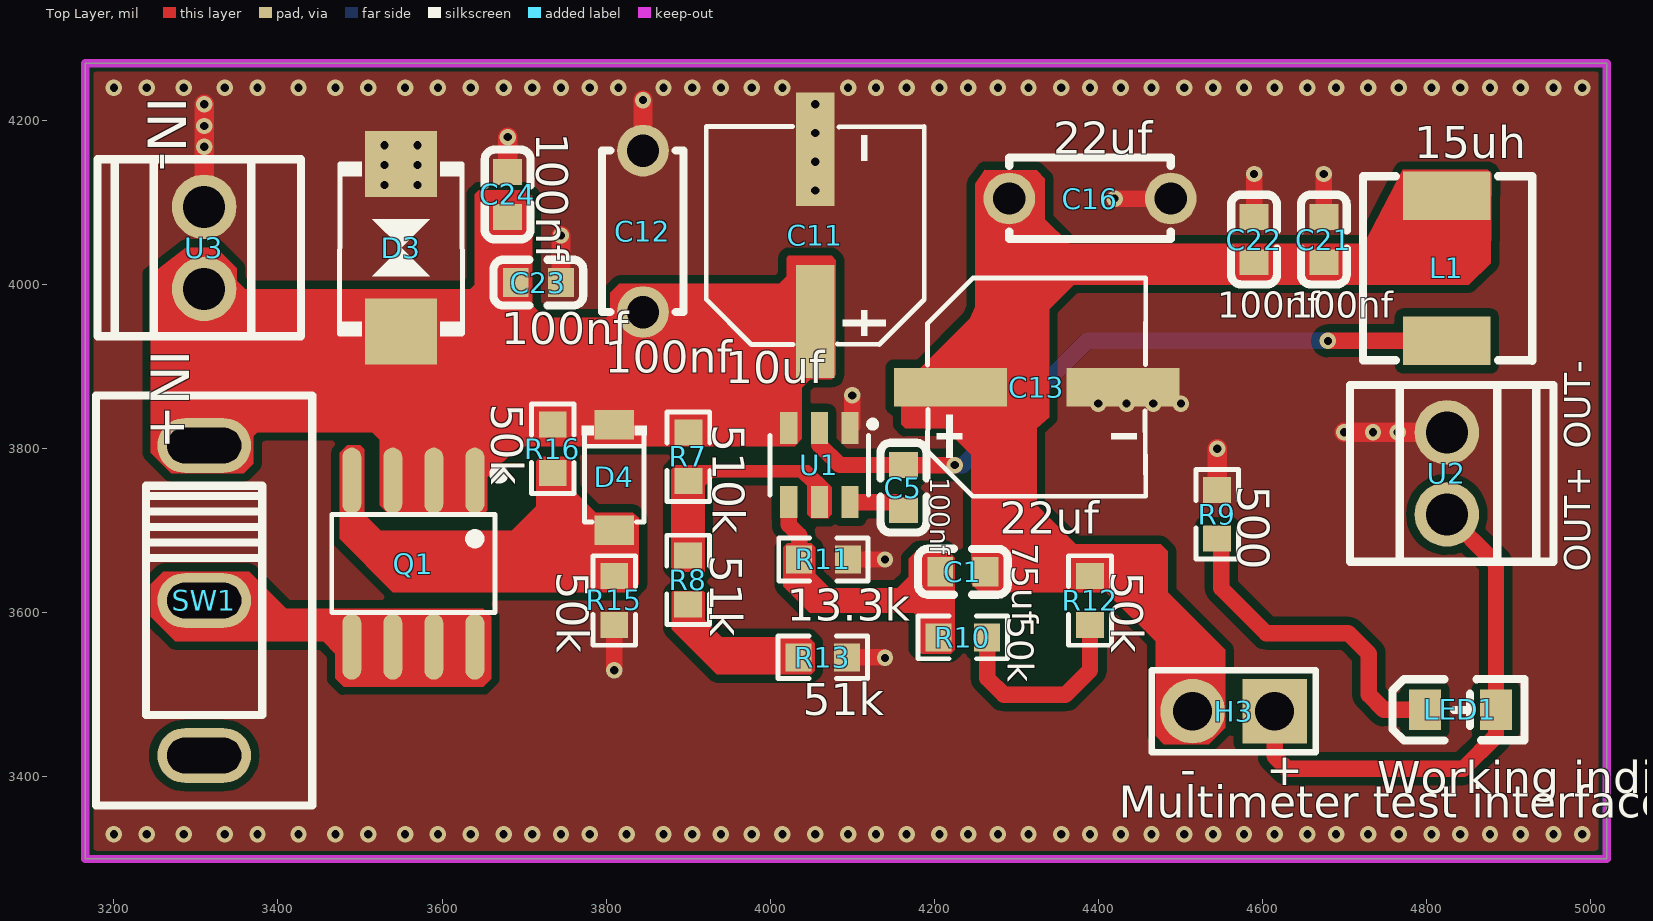
[diagram p0: Top Layer view]
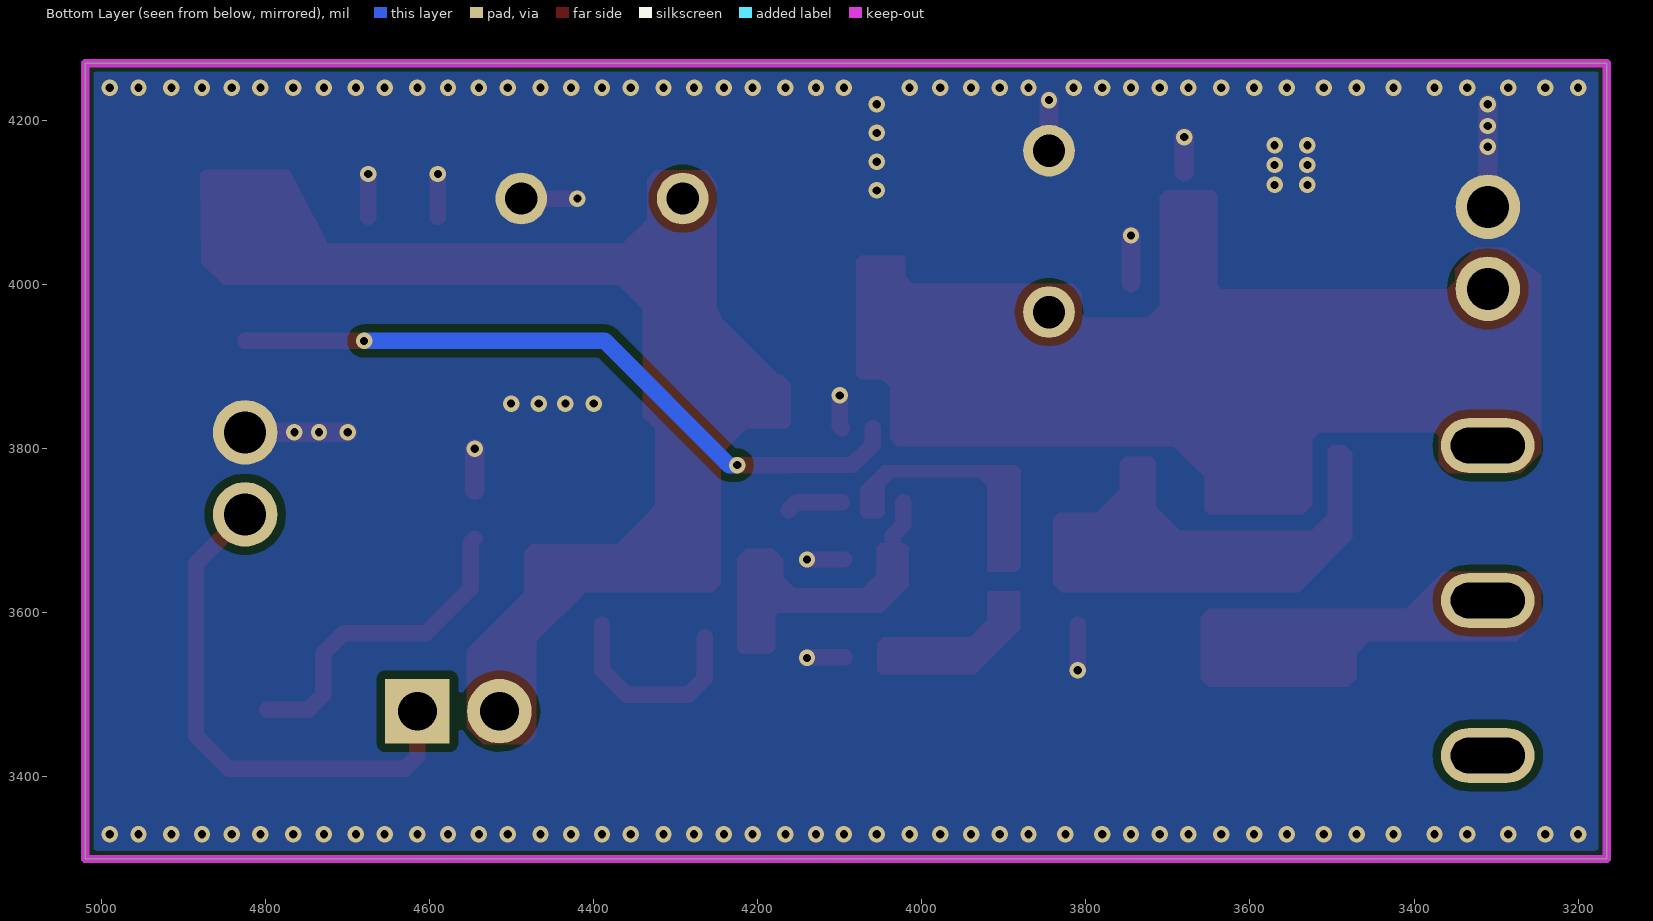
[diagram p1: Bottom Layer view, seen from below]
# Altium PCB MISC52037.pcbdoc
Units mil, origin at the board's own origin, x right, y up, seen from the top; angles counter-clockwise.
Board outline 1855 x 970 mil, 2 copper layers (Top Layer, Bottom Layer), stack 62.206 mil thick; 29 components, 13 nets, 69 pads, 126 vias.

## Layer stack, top to bottom
Top Solder Mask Layer: solder mask 0.394, Dk 3.3
Top Layer: signal copper 1.379
Dielectric1: surface 59.449, FR4, Dk 4.5
Bottom Layer: signal copper 1.378
Bottom Solder Mask Layer: solder mask 0.394, Dk 3.3

## Board outline
3165,4270 3165,3300 5020,3300 5020,4270

## Design rules (kind name [scope] priority, off if disabled: settings)
BoardOutlineClearance copperThickness2oz_1 [All] p2 off: genericclearance=7.99 ignorepadtopadclearanceinfootprint=FALSE except(0: Arc-SplitContinuation Track-SplitContinuation SMDPad-SplitContinuation THPad-SplitContinuation Via-SplitContinuation Fill-SplitContinuation Region-SplitContinuation Poly-SplitContinuation Text-SplitContinuation Hole-SplitContinuation; 5.98: Arc-CutoutEdge SMDPad-CutoutEdge THPad-CutoutEdge Via-CutoutEdge Fill-CutoutEdge Region-CutoutEdge Text-CutoutEdge; 6.93: Hole-OutlineEdge Hole-CutoutEdge; 10: Poly-OutlineEdge Poly-CutoutEdge; 11.81: Arc-OutlineEdge Track-OutlineEdge SMDPad-OutlineEdge THPad-OutlineEdge Via-OutlineEdge Fill-OutlineEdge Region-OutlineEdge Text-OutlineEdge Track-CutoutEdge)
BoardOutlineClearance Plane_innerPlane_1 [All] p4 off: genericclearance=6 ignorepadtopadclearanceinfootprint=FALSE except(0: Arc-SplitContinuation Track-SplitContinuation SMDPad-SplitContinuation THPad-SplitContinuation Via-SplitContinuation Fill-SplitContinuation Region-SplitContinuation Poly-SplitContinuation Text-SplitContinuation Hole-SplitContinuation; 6: SMDPad-CutoutEdge THPad-CutoutEdge Via-CutoutEdge Fill-CutoutEdge Region-CutoutEdge Text-CutoutEdge; 6.93: Hole-OutlineEdge Hole-CutoutEdge; 10: Poly-OutlineEdge Poly-CutoutEdge; 11.8: Arc-OutlineEdge Track-OutlineEdge SMDPad-OutlineEdge THPad-OutlineEdge Via-OutlineEdge Fill-OutlineEdge Region-OutlineEdge Text-OutlineEdge; 11.81: Arc-CutoutEdge Track-CutoutEdge)
BoardOutlineClearance Copper_copperRegion_1 [All] p6 off: genericclearance=6 ignorepadtopadclearanceinfootprint=FALSE except(0: Arc-SplitContinuation Track-SplitContinuation SMDPad-SplitContinuation THPad-SplitContinuation Via-SplitContinuation Fill-SplitContinuation Region-SplitContinuation Poly-SplitContinuation Text-SplitContinuation Hole-SplitContinuation; 6: SMDPad-CutoutEdge THPad-CutoutEdge Via-CutoutEdge Fill-CutoutEdge Region-CutoutEdge Text-CutoutEdge; 6.93: Hole-OutlineEdge Hole-CutoutEdge; 10: Poly-OutlineEdge Poly-CutoutEdge; 11.8: Arc-OutlineEdge Track-OutlineEdge SMDPad-OutlineEdge THPad-OutlineEdge Via-OutlineEdge Fill-OutlineEdge Region-OutlineEdge Text-OutlineEdge; 11.81: Arc-CutoutEdge Track-CutoutEdge)
BoardOutlineClearance copperThickness1oz_1 [All] p8: genericclearance=6 ignorepadtopadclearanceinfootprint=FALSE except(0: Arc-SplitContinuation Track-SplitContinuation SMDPad-SplitContinuation THPad-SplitContinuation Via-SplitContinuation Fill-SplitContinuation Region-SplitContinuation Poly-SplitContinuation Text-SplitContinuation Hole-SplitContinuation; 6: SMDPad-CutoutEdge THPad-CutoutEdge Via-CutoutEdge Fill-CutoutEdge Region-CutoutEdge Text-CutoutEdge; 6.93: Hole-OutlineEdge Hole-CutoutEdge; 10: Poly-OutlineEdge Poly-CutoutEdge; 11.8: Arc-OutlineEdge Track-OutlineEdge SMDPad-OutlineEdge THPad-OutlineEdge Via-OutlineEdge Fill-OutlineEdge Region-OutlineEdge Text-OutlineEdge; 11.81: Arc-CutoutEdge Track-CutoutEdge)
Clearance copperThickness2oz [All] p1 off: gap=7.99 ignorepadtopadclearanceinfootprint=FALSE except(5.98: SMDPad-Track SMDPad-SMDPad THPad-Track SMDPad-THPad THPad-THPad Track-Via SMDPad-Via THPad-Via Via-Via Fill-Track Region-Track Fill-SMDPad Region-SMDPad Fill-THPad Region-THPad Fill-Via Region-Via Fill-Fill Fill-Region Region-Region Arc-Track Arc-SMDPad Arc-THPad Arc-Via Fill-Arc Region-Arc Arc-Arc Text-Track SMDPad-Text Text-THPad Text-Via Fill-Text Region-Text Arc-Text Text-Text; 6.93: Hole-Track Hole-SMDPad Hole-THPad Hole-Via Fill-Hole Region-Hole Hole-Arc Hole-Text; 10: Poly-Track Poly-SMDPad Poly-THPad Poly-Via Poly-Fill Poly-Region Poly-Poly Poly-Arc Poly-Text Poly-Hole)
Clearance Plane_innerPlane [All] p3 off: gap=6 ignorepadtopadclearanceinfootprint=FALSE except(5.98: SMDPad-Track SMDPad-SMDPad THPad-Track SMDPad-THPad THPad-THPad Track-Via SMDPad-Via THPad-Via Via-Via Fill-Track Region-Track Fill-SMDPad Region-SMDPad Fill-THPad Region-THPad Fill-Via Region-Via Fill-Fill Fill-Region Region-Region; 6.93: Hole-Track Hole-SMDPad Hole-THPad Hole-Via Fill-Hole Region-Hole Hole-Arc Hole-Text; 10: Poly-Track Poly-SMDPad Poly-THPad Poly-Via Poly-Fill Poly-Region Poly-Poly Poly-Arc Poly-Text Poly-Hole)
Clearance Copper_copperRegion [All] p5 off: gap=6 ignorepadtopadclearanceinfootprint=FALSE except(5.98: SMDPad-Track SMDPad-SMDPad THPad-Track SMDPad-THPad THPad-THPad Track-Via SMDPad-Via THPad-Via Via-Via Fill-Track Region-Track Fill-SMDPad Region-SMDPad Fill-THPad Region-THPad Fill-Via Region-Via Fill-Fill Fill-Region Region-Region; 6.93: Hole-Track Hole-SMDPad Hole-THPad Hole-Via Fill-Hole Region-Hole Hole-Arc Hole-Text; 10: Poly-Track Poly-SMDPad Poly-THPad Poly-Via Poly-Fill Poly-Region Poly-Poly Poly-Arc Poly-Text Poly-Hole)
Clearance copperThickness1oz [All] p7: gap=6 ignorepadtopadclearanceinfootprint=FALSE except(5.98: SMDPad-Track SMDPad-SMDPad THPad-Track SMDPad-THPad THPad-THPad Track-Via SMDPad-Via THPad-Via Via-Via Fill-Track Region-Track Fill-SMDPad Region-SMDPad Fill-THPad Region-THPad Fill-Via Region-Via Fill-Fill Fill-Region Region-Region; 6.93: Hole-Track Hole-SMDPad Hole-THPad Hole-Via Fill-Hole Region-Hole Hole-Arc Hole-Text; 10: Poly-Track Poly-SMDPad Poly-THPad Poly-Via Poly-Fill Poly-Region Poly-Poly Poly-Arc Poly-Text Poly-Hole)
DiffPairsRouting differentialPair [All] p1: maxlimit=6 minlimit=6 mostfreqgap=6 toplayer_minwidth=5 toplayer_prefwidth=10 toplayer_maxwidth=100 toplayer_mingap=6 toplayer_prefgap=6 toplayer_maxgap=6 bottomlayer_minwidth=5 bottomlayer_prefwidth=10 bottomlayer_maxwidth=100 bottomlayer_mingap=6 bottomlayer_prefgap=6 bottomlayer_maxgap=6 maxuncoupledlength=10
HoleToHoleClearance otherClearance [All] p1: gap=11.81 allowstackedmicrovias=TRUE
Length netLength [All] p1: minlimit=0 maxlimit=0
PasteMaskExpansion pasteMaskExpansion [All] p1: expansion=0
PlaneConnect innerPlane [All] p1: planeconnectstyle=Relief reliefexpansion=20 reliefentries=4 reliefconductorwidth=10 reliefairgap=10
PolygonConnect copperRegion [All] p1: connectstyle=Direct reliefconductorwidth=10 reliefentries=4 polygonreliefangle="90 Angle" airgapwidth=10 via.connectstyle=Relief via.reliefconductorwidth=10 via.reliefentries=4 via.polygonreliefangle="90 Angle" via.airgapwidth=10
RoutingVias viaSize [All] p1: holewidth=10 width=20 viastyle="Through Hole" minholewidth=9 minwidth=19.68 maxholewidth=248.03 maxwidth=393.7
SolderMaskExpansion solderMaskExpansion [IsVia] p1: expansion=-1000 istentingtop=TRUE
SolderMaskExpansion solderMaskExpansion [All] p2: expansion=2 istentingtop=FALSE
Width copperThickness2oz_2 [All] p1 off: maxlimit=100 minlimit=8 preferedwidth=10
Width copperThickness1oz_2 [All] p2: maxlimit=100 minlimit=5 preferedwidth=20

## Components (designator, comment, footprint, x,y, rotation, side; value= is the part's Value field where it differs from the comment)
C1 "75uf" C0603 4235,3650 r0 top
C5 "0.1uf" C0603 4162.56,3752.56 r270 top
C11 "10uf" CAP-SMD_BD6.3-L6.6-W6.6-FD 4055,4060 r90 top
C12 "100nf" CAP-TH_L5.0-W2.5-P5.00-D1.0 3845,4065 r270 top
C13 "22uf" CAP-SMD_BD6.3-L6.6-W6.6-FD 4325,3875 r0 top
C16 "22uf" CAP-TH_L5.0-W2.5-P5.00-D1.0 4390,4105 r180 top
C21 "0.1uf" C0603 4675,4055 r90 top
C22 "0.1uf" C0603 4590,4055 r90 top
C23 "100nf" C0603 3717.44,4002.56 r0 top
C24 "100nf" C0603 3680,4110 r90 top
D3 "SMBJ28CA" SMB_L4.6-W3.6-LS5.4-BI 3550,4045 r270 top
D4 "BZT52C12" SOD-123_L2.7-W1.6-LS3.7-RD 3810,3765 r270 top
H3 "PZ254V-11-02P" HDR-TH_2P-P2.54-V-M 4565,3480 r180 top
L1 "15uH" IND-SMD_L5.7-W5.2_GSM0530 4825,4020 r90 top
LED1 "NCD0805R1" LED0805-RD 4841.62,3481.62 r0 top
Q1 "AO4421" SOIC-8_L4.9-W3.9-P1.27-LS6.0-BL 3565,3660 r180 top
R7 "510kΩ" R0603 3900.34,3790.34 r90 top
R8 "51kΩ" R0603 3900,3640 r90 top
R9 "500Ω" R0603 4545,3720 r270 top
R10 "50kΩ" R0603 4235,3570 r0 top
R11 "13.3kΩ" R0603 4065,3665 r180 top
R12 "50kΩ" R0603 4390,3615 r90 top
R13 "51kΩ" R0603 4064.32,3545.68 r180 top
R15 "50kΩ" R0603 3810,3615 r90 top
R16 "50kΩ" R0603 3735,3800 r90 top
SW1 "SS12D10G4 071" SW-TH_SHOU-HAN_SS12D10G4 3310,3615 r270 top
U1 "GD30DC1354" SOT-23-6_L2.9-W1.7-P0.95-LS2.8-BL 4060,3780 r180 top
U2 "KF128-2.54-2P" CONN-TH_P2.54_KF128-2.54-2P 4825,3770 r90 top
U3 "KF128-2.54-2P" CONN-TH_P2.54_KF128-2.54-2P 3310,4045 r270 top

## Footprints (in the part's own frame and the unit in brackets; to place one, negate y for a bottom-side part, rotate by r counter-clockwise, add the part's x,y. Pads: shape width x height; smd on the part's side, far side on the other; paste and mask are expansions set on the pad)
C0603 [mm]
  rect 0.8x0.9 smd: 1(-0.7,0) 2(0.7,0)
  silkscreen extent -1.39,-0.71 1.39,0.71
CAP-SMD_BD6.3-L6.6-W6.6-FD [mm]
  rect 3.5x1.2 smd: 1(-2.67,0) 2(2.67,0)
  silkscreen extent -3.38,-3.38 3.38,3.38
CAP-TH_L5.0-W2.5-P5.00-D1.0 [mm]
  round 1.6 hole 1: 1(-2.5,0) 2(2.5,0)
  silkscreen extent -2.5,-1.27 2.5,1.25
CONN-TH_P2.54_KF128-2.54-2P [mm]
  round 2 hole 1.3: 1(-1.27,0) 2(1.27,0)
  silkscreen extent -2.74,-3.3 2.74,3
HDR-TH_2P-P2.54-V-M [mm]
  rect 2x2 hole 1.2: 1(-1.27,0)
  round 2 hole 1.2: 2(1.27,0)
  silkscreen extent -2.54,-1.27 2.54,1.27
IND-SMD_L5.7-W5.2_GSM0530 [mm]
  rect 1.5x2.7 smd: 1(-2.25,0) 2(2.25,0)
  silkscreen extent -2.86,-2.64 2.85,2.6
LED0805-RD [mm]
  rect 1x1.25 smd: 1(-1.1,0) 2(1.1,0)
  silkscreen extent -2.1,-0.95 1.98,0.96
R0603 [mil]
  rect 31.75x34.02 smd paste-3937.01 mask+2: 1(-29.66,0) 2(29.66,0)
  silkscreen extent -55,-26 55,26
SMB_L4.6-W3.6-LS5.4-BI [mil]
  rect 80.61x88.23 smd: 1(-102.02,0) 2(102.02,0)
  silkscreen extent -105,-75 108,75
SOD-123_L2.7-W1.6-LS3.7-RD [mm]
  rect 0.91x1.22 smd: 1(-1.635,0) 2(1.635,0)
  silkscreen extent -1.6,-1 1.38,1
SOIC-8_L4.9-W3.9-P1.27-LS6.0-BL [mm]
  oval 0.588x2.045 smd: 1(-1.905,-2.57) 2(-0.635,-2.57) 3(0.635,-2.57) 4(1.905,-2.57) 5(1.905,2.57) 6(0.635,2.57) 7(-0.635,2.57) 8(-1.905,2.57)
  silkscreen extent -2.8,-2.92 2.53,1.52
SOT-23-6_L2.9-W1.7-P0.95-LS2.8-BL [mm]
  rect 0.532x0.99 smd paste+0 mask+0.102: 1(-0.95,-1.145) 2(0,-1.145) 3(0.95,-1.145) 4(0.95,1.145) 5(0,1.145) 6(-0.95,1.145)
  silkscreen extent -1.75,-1.37 1.53,0.93
SW-TH_SHOU-HAN_SS12D10G4 [mm]
  oval 1.7x2.9 hole 1.1 slot 2.3 at 90 deg paste+0 mask+0.05: 1(-4.8,0) 2(0,0) 3(4.8,0)
  silkscreen extent -6.35,-3.35 6.35,3.35

## Via types
v1: diameter 20, hole 10, Top Layer to Bottom Layer, 126 vias

## Nets (pads, with @x,y where several pads share a name; then routed paths per layer and width w, separated by ;. In a path a pad name is that pad's centre, name@x,y a point inside that pad or via, vN(x,y) a via of type N, cw(c..) or ccw(c..) an arc to the next point about the centre after c; other vN are vias at no path point)
24V: C11.1 C12.2 C23.1 C24.1 D3.2 D4.1 Q1.1 Q1.2 Q1.3 R7.2 R16.2 SW1.1 U1.3 U3.2
$1N1: Q1.5 Q1.6 Q1.7 Q1.8 SW1.2
$1N10: LED1.1 R9.2 | length 401.5
  Top Layer w20: R9.2 4550,3685.34 4550,3630 4605,3575 4705,3575 4730,3550 4730,3500 4748.38,3481.62 LED1.1
$1N13: R7.1 R8.2 U1.5
$1N14: C5.2 U1.6 | length 69.3
  Top Layer w20: U1.6 4152.64,3734.92 C5.2
$1N17: C1.2 C13.1 C16.2 C21.1 C22.1 H3.2 L1.2 R12.2
$1N19: R10.2 R12.1 | length 251.2
  Top Layer w20: R10.2 4264.66,3520.34 4285,3500 4360,3500 4390,3530 R12.1
$1N20: C1.1 R10.1 R11.2 U1.4 | length 75.2
  Top Layer w20: U1.4 4022.6,3707.4 4035.34,3694.66 R11.2
$1N41: C5.1 L1.1 U1.2 | length 858.2
  Top Layer w20: U1.2 4060,3805 4084.88,3780.12 C5.1 4162.68,3780 v1(4225,3780) ; v1(4680,3931.41) L1.1
  Bottom Layer w20: v1(4225,3780) 4235,3780 4386.41,3931.41 v1(4680,3931.41)
$1N48: D4.2 Q1.4 R15.2 R16.1
$1N50: R8.1 R13.2
+5V: H3.1 LED1.2 U2.1 | length 642.6
  Top Layer w20: H3.1 4615,3425 4630,3410 4845,3410 4884.93,3449.93 LED1.2 4884.93,3660.07 U2.1
GND: C11.2 C12.1 C13.2 C16.1 C21.2 C22.2 C23.2 C24.2 D3.1 R9.1 R11.1 R13.1 R15.1 U1.1 U2.2 U3.1 | length 823
  Top Layer w20: v1(3810,3530) R15.1 ; R13.1 4139.32,3545.68 v1(4140,3545) ; R11.1 v1(4140,3665) ; U1.1 4100,3827.68 v1(4100,3865) ; v1(4420,4105) C16.1 ; C22.2 v1(4590,4135) ; C21.2 v1(4675,4135)
  Top Layer w23.62: U3.1 v1(3310,4168.09) v1(3310,4193.46) v1(3310,4220) ; C24.2 v1(3680,4180) ; C23.2 v1(3745,4060) ; C12.1 v1(3845,4225) ; R9.1 v1(4545,3800) ; v1(4700.02,3820.02) v1(4735,3820) v1(4765,3820) U2.2
  other v1: 3200,3330 3240,3330 3285,3330 3335,3330 3375,3330 3425,3330 3470,3330 3510,3330 3555,3330 3595,3330 3635,3330 3675,3330 3710,3330 3745,3330 3780,3330 3825,3330 3870,3330 3905,3330 3940,3330 3977.68,3330 4015,3330 4055,3330 4095,3330 4129.07,3330 4166.39,3330 4206.39,3330 4241.39,3330 4277.68,3330 4315,3330 4355,3330 4390,3330 4427.68,3330 4465,3330 4505,3330 4540,3330 4577.68,3330 4615,3330 4655,3330 4690,3330 4729.07,3330 4766.39,3330 4806.39,3330 4841.39,3330 4877.68,3330 4915,3330 4955,3330 4990,3330 4400.07,3855 4434.56,3855 4467.13,3855.01 4500.78,3855.01 4055,4115 3530,4121.71 3570,4121.71 3530,4145.9 3570,4145.9 4055,4150 3530,4170 3570,4170 4055,4185 4055,4220 3200,4240 3240,4240 3285,4240 3335,4240 3375,4240 3425,4240 3470,4240 3510,4240 3555,4240 3595,4240 3635,4240 3675,4240 3710,4240 3745,4240 3780,4240 3815,4240 3870,4240 3905,4240 3940,4240 3977.68,4240 4015,4240 4095,4240 4129.07,4240 4166.39,4240 4206.39,4240 4241.39,4240 4277.68,4240 4315,4240 4355,4240 4390,4240 4427.68,4240 4465,4240 4505,4240 4540,4240 4577.68,4240 4615,4240 4655,4240 4690,4240 4729.07,4240 4766.39,4240 4806.39,4240 4841.39,4240 4877.68,4240 4915,4240 4955,4240 4990,4240
pads on no net: SW1.3

## Polygon pours and split planes (outlines as drawn)
GND on Top Layer (solid, remove dead copper, pour order 0): 3070,4355 3070,3075 5160,3075 5160,4355
GND on Bottom Layer (solid, remove dead copper, pour order 2): 3000,4425 3000,3000 5255,3000 5255,4425

## Keep-outs
Board Outline Layer:
  the board outline again, w10

## Other copper
Top Layer:
  region net 24V: 3245,3795 3245,4012.31 3287.37,4045 3325,4045 3350,4020 3350,4005 3360.33,3994.67 3635,3995 3640,4000 3640,4110 3645,4115 3702.94,4115 3710,4107.94 3710,3975 3725,3960 3800,3960 3805,3965 3805,3990 3816.23,4001.23 4011.23,4001.23 4020,4010 4020,4032.94 4022.06,4035 4075,4035 4080,4030 4080,3890 4075,3885 4049.07,3885 4038.56,3874.49 4038.56,3812.09 4029.76,3803.29 3693.29,3803.29 3655,3765 3655,3725.04 3649.98,3720.02 3534.98,3720.02 3524.16,3730.84 3524.16,3810.83 3514.99,3820 3375.02,3820 3370,3814.98 3370,3781.67 3358.33,3770 3270,3770
  region net $1N1: 3650,3510 3480,3510 3470,3520 3470,3550 3455,3565 3275,3565 3245,3595 3245,3635 3260,3650 3365,3650 3410,3605 3650,3605 3659.83,3595.17 3659.83,3519.83
  region net $1N20: 4015.98,3680 4020.98,3685 4050,3685 4055,3680 4055,3647.8 4072.8,3630 4155,3630 4169.06,3644.06 4169.06,3665.76 4181.26,3677.96 4214.29,3677.96 4225,3667.25 4225,3555 4220,3550 4185,3550 4178.95,3556.05 4178.95,3596.05 4175,3600 4048.37,3600 4015.98,3632.39
  region net $1N13: 4045,3720 4045,3755 4034.59,3765.41 3930.41,3765.41 3920,3755 3920,3650 3884.63,3650 3879.63,3655 3879.63,3774.63 3885,3780 4047.76,3780 4075,3752.76 4075,3720 4071.47,3716.47 4071.47,3715 4050,3715
  region net $1N50: 3881.42,3626.42 3918.58,3626.42 3920,3625 3920,3591.48 3941.01,3570.47 4046.99,3570.47 4054.32,3563.13 4054.32,3529.32 4050,3525 3935,3525 3880,3580 3880,3625
  region net $1N48: 3500,3804.21 3505,3799.21 3505,3720 3525,3700 3685,3700 3715,3730 3715,3785 3720,3790 3751.98,3790 3758.53,3783.45 3758.53,3750.84 3787.43,3721.94 3832.67,3721.94 3840,3715.82 3840,3635 3830,3625 3540,3625 3475,3690 3475,3795 3484.21,3804.21
  region net $1N17: 4245,3635.53 4245,3792.69 4212.6,3825.1 4164.9,3825.1 4160,3830 4160,3880 4170,3890 4175.5,3890 4175.86,3890.86 4244.14,3959.14 4250,3973.28 4250,4123.1 4261.79,4140 4324.82,4139.61 4335,4129.43 4335,4080 4365,4050 4724.16,4050 4771.31,4140 4875,4140 4879.94,4135.06 4878.73,4025.88 4851.54,4000 4370,4000 4340,3970 4340,3838.12 4325,3825 4325,3730.97 4372.45,3683.52 4476.48,3683.52 4485,3675 4485,3625 4555,3555 4555,3460 4535,3440 4480,3440 4470,3450 4470,3565 4410,3625 4255.54,3625

## Silkscreen, mask and mechanical layers (free items; w line width, h text height)
Top Silkscreen Layer:
  text "IN-" at 3241.4,4228.35 h47.24 r270
  text "100nf" at 3715,4185 h39.37 r270
  text "22uf" at 4345,4159.78 h39.37
  text "15uh" at 4785,4154.42 h39.37
  text "100nf" at 4545,3960 h31.5
  text "100nf" at 4635,3960 h31.5
  text "100nf" at 3672.44,3927.44 h39.37
  text "IN+" at 3245,3920 h47.24 r270
  text "100nf" at 3798.63,3892.51 h39.37
  text "10uf" at 3945,3880 h39.37
  text "50k" at 3660,3855 h39.37 r270
  text "510k" at 3930,3830 h39.37 r270
  text "OUT-" at 5000,3800 h31.5 r90
  text "100nf" at 4195,3765 h23.62 r270
  text "500" at 4570,3755 h39.37 r270
  text "22uf" at 4280,3696.15 h39.37
  text "75uf" at 4295,3685 h31.5 r270
  text "51k" at 3927.28,3670 h39.37 r270
  text "50k" at 3740,3650 h39.37 r270
  text "50k" at 4415.61,3650 h39.37 r270
  text "OUT+" at 5000,3650 h31.5 r90
  text "50k" at 4290,3595 h31.5 r270
  text "13.3k" at 4020,3590 h39.37
  text "51k" at 4040,3475 h39.37
  text "-" at 4500,3390 h39.37
  text "+" at 4605,3390 h39.37
  text "Working indicator light" at 4740,3380 h39.37
  text "Multimeter test interface" at 4425,3350 h39.37